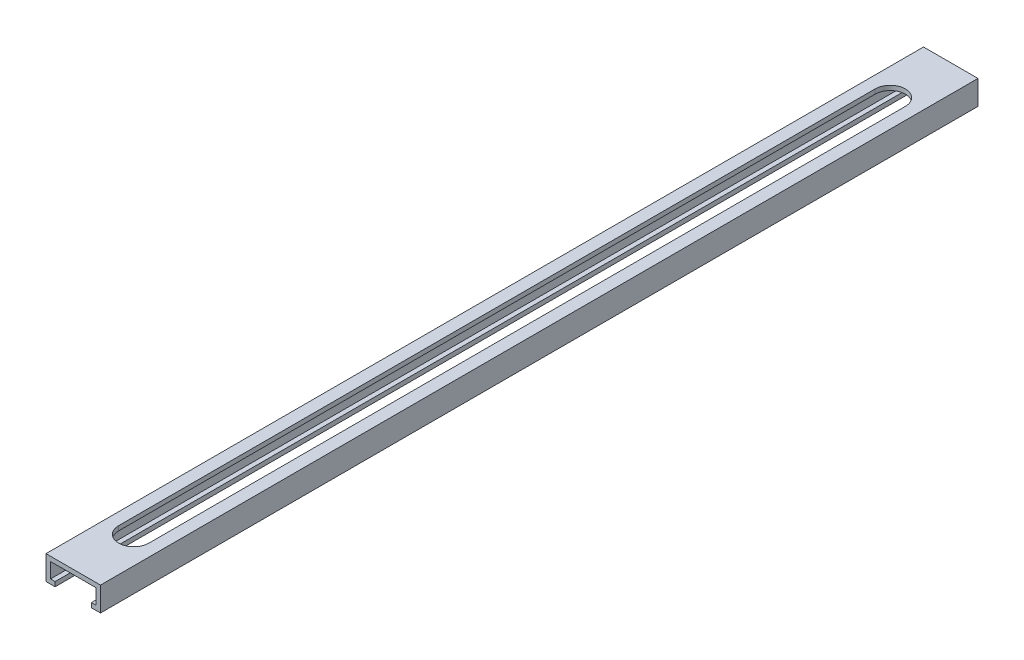
SolidWorks part; units mm, degrees
ref_plane "Front Plane" through (0, 0, 0) normal (0, 0, 1) x (1, 0, 0)
ref_plane "Top Plane" through (0, 0, 0) normal (0, 1, 0) x (1, 0, 0)
ref_plane "Right Plane" through (0, 0, 0) normal (1, 0, 0) x (0, 0, -1)
ref_plane "Plane1" through (0, 13, 0) normal (0, 1, 0) x (1, 0, 0)
sketch "Sketch1" plane through (0, 13, 0) normal (0, 1, 0) x (1, 0, 0)
  line L0 (-18, -290) -> (18, -290)
  line L1 (18, -290) -> (18, 290)
  line L2 (18, 290) -> (-18, 290)
  line L3 (-18, 290) -> (-18, -290)
extrude "Boss-Extrude1" add sketch "Sketch1" against normal blind 16
sketch "Sketch2" plane through (0, 0, -290) normal (0, 0, -1) x (-1, 0, 0)
  line L0 (12, -3) -> (12, 0)
  line L1 (12, 0) -> (15, 0)
  line L2 (15, 0) -> (15, 10)
  line L3 (15, 10) -> (-15, 10)
  line L4 (-15, 10) -> (-15, 0)
  line L5 (-15, 0) -> (-12, 0)
  line L6 (-12, 0) -> (-12, -3)
  line L7 (-12, -3) -> (12, -3)
extrude "Cut-Extrude1" cut sketch "Sketch2" against normal through all
sketch "Sketch3" plane through (0, 10, 0) normal (0, -1, 0) x (1, 0, 0)
  line L0 (10, -250) -> (10, 250)
  line L1 (-10, 250) -> (-10, -250)
  arc A0 (-10, -250) -> (10, -250) centre (0, -250) ccw
  arc A1 (10, 250) -> (-10, 250) centre (0, 250) ccw
extrude "Cut-Extrude2" cut sketch "Sketch3" against normal through all
